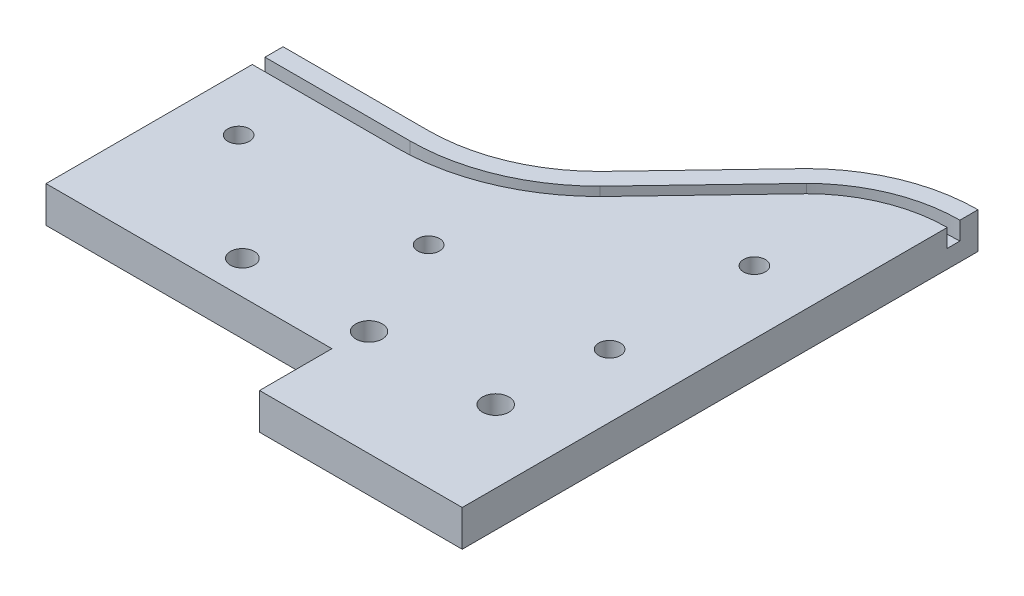
from build123d import *

# Parameters (mm, degrees)
EXTRUDE_1_DEPTH      = 20
CUT_EXTRUDE_1_DEPTH  = 10
SKETCH_4_W           = 45
SKETCH_4_H           = 90
CUT_EXTRUDE_2_DEPTH  = 5
SKETCH_5_W           = 112
SKETCH_5_H           = 20
EXTRUDE_2_DEPTH      = 40
CUT_EXTRUDE_3_REACH  = 1227.871
SKETCH_6_R           = 6
SKETCH_6_R_2         = 5
CUT_EXTRUDE_4_REACH  = 1228.116
SKETCH_7_R           = 7.332886018
SKETCH_7_R_2         = 7.301331484
SKETCH_7_R_3         = 6.603217824
SKETCH_24_R          = 6
CUT_EXTRUDE_21_DEPTH = 25


with BuildPart() as part:
    # 草图1 → 凸台-拉伸1 (new body)
    with BuildSketch(Plane(origin=(0, 0, 0), x_dir=(1, 0, 0), z_dir=(0, 1, 0))):
        with BuildLine():
            Line((-190, -173.659488393), (0, -173.659488393))
            Line((0, -173.659488393), (0, 71.340511607))
            ThreePointArc((0, 71.340511607), (-36.354926075, 64.109067196), (-67.175144213, 43.51565582))
            add(Edge.make_bspline(
                [(-122.824855787, -14.834632605), (-95, 14.340511607), (-67.175144213, 43.51565582)],
                knots=[0, 0, 0, 1, 1, 1], degree=2))
            ThreePointArc((-122.824855787, -14.834632605), (-153.645073925, -35.428043981), (-190, -42.659488393))
            Line((-190, -42.659488393), (-270, -42.659488393))
            Line((-270, -42.659488393), (-270, -173.659488393))
            Line((-270, -173.659488393), (-190, -173.659488393))
        make_face()
    extrude(amount=EXTRUDE_1_DEPTH)

    # 草图2 → 切除-拉伸1 (cut)
    with BuildSketch(Plane(origin=(0, 20, 0), x_dir=(1, 0, 0), z_dir=(0, 1, 0))):
        with BuildLine():
            Line((-270, -52.659488393), (-190, -52.659488393))
            ThreePointArc((-190, -52.659488393), (-149.762170559, -44.64359576), (-115.668000558, -21.819813762))
            Line((-115.668000558, -21.819813762), (-60.022606457, 36.52594767))
            ThreePointArc((-60.022606457, 36.52594767), (-32.474897495, 54.892284551), (0, 61.340511607))
            Line((0, 61.340511607), (0, 54.340511607))
            ThreePointArc((0, 54.340511607), (-29.760862596, 48.439686759), (-55.01881141, 31.630025903))
            Line((-55.01881141, 31.630025903), (-110.655962205, -26.707092192))
            ThreePointArc((-110.655962205, -26.707092192), (-147.042646878, -51.093843482), (-190, -59.659488393))
            Line((-190, -59.659488393), (-270, -59.659488393))
            Line((-270, -59.659488393), (-270, -52.659488393))
        make_face()
    extrude(amount=-CUT_EXTRUDE_1_DEPTH, mode=Mode.SUBTRACT)

    # 草图4 → 切除-拉伸2 (cut)
    with BuildSketch(Plane.XZ):
        with Locations((-247.5, 99.659488393)):
            Rectangle(SKETCH_4_W, SKETCH_4_H)
    extrude(amount=-CUT_EXTRUDE_2_DEPTH, mode=Mode.SUBTRACT)

    # 草图5 → 凸台-拉伸2 (add)
    with BuildSketch(Plane.XY.offset(173.659488393)):
        with Locations((-56, 10)):
            Rectangle(SKETCH_5_W, SKETCH_5_H)
    extrude(amount=EXTRUDE_2_DEPTH)

    # 切除-拉伸3: up to this face of the body (flat: up to its plane)
    cut_extrude_3_end = Plane(part.part.faces().sort_by_distance((-99.039367246, 0, 91.650022184))[0])
    # 草图6 → 切除-拉伸3 (cut, up to the picked face)
    with BuildSketch(Plane(origin=(600.126281628, 25, -649.482989384), x_dir=(0, 0, -1), z_dir=(0, 1, 0)), mode=Mode.PRIVATE) as cut_extrude_3_sk1:
        with Locations(Location((-666.704267343, 635.126281628, 0), (0, 0, 180))):
            Circle(SKETCH_6_R)
    cut_extrude_3_tool1 = split(extrude(cut_extrude_3_sk1.sketch, amount=-CUT_EXTRUDE_3_REACH, mode=Mode.PRIVATE), bisect_by=cut_extrude_3_end, keep=Keep.BOTH, mode=Mode.PRIVATE)
    # 草图6 → 切除-拉伸3 (cut, up to the picked face)
    with BuildSketch(Plane(origin=(600.126281628, 25, -649.482989384), x_dir=(0, 0, -1), z_dir=(0, 1, 0)), mode=Mode.PRIVATE) as cut_extrude_3_sk2:
        with Locations(Location((-746.704267343, 635.126281628, 0), (0, 0, 180))):
            Circle(SKETCH_6_R_2)
    cut_extrude_3_tool2 = split(extrude(cut_extrude_3_sk2.sketch, amount=-CUT_EXTRUDE_3_REACH, mode=Mode.PRIVATE), bisect_by=cut_extrude_3_end, keep=Keep.BOTH, mode=Mode.PRIVATE)
    # 草图6 → 切除-拉伸3 (cut, up to the picked face)
    with BuildSketch(Plane(origin=(600.126281628, 25, -649.482989384), x_dir=(0, 0, -1), z_dir=(0, 1, 0)), mode=Mode.PRIVATE) as cut_extrude_3_sk3:
        with Locations(Location((-746.704267343, 840.126281628, 0), (0, 0, 180))):
            Circle(SKETCH_6_R)
    cut_extrude_3_tool3 = split(extrude(cut_extrude_3_sk3.sketch, amount=-CUT_EXTRUDE_3_REACH, mode=Mode.PRIVATE), bisect_by=cut_extrude_3_end, keep=Keep.BOTH, mode=Mode.PRIVATE)
    # 草图6 → 切除-拉伸3 (cut, up to the picked face)
    with BuildSketch(Plane(origin=(600.126281628, 25, -649.482989384), x_dir=(0, 0, -1), z_dir=(0, 1, 0)), mode=Mode.PRIVATE) as cut_extrude_3_sk4:
        with Locations(Location((-746.704267343, 735.126281628, 0), (0, 0, 180))):
            Circle(SKETCH_6_R)
    cut_extrude_3_tool4 = split(extrude(cut_extrude_3_sk4.sketch, amount=-CUT_EXTRUDE_3_REACH, mode=Mode.PRIVATE), bisect_by=cut_extrude_3_end, keep=Keep.BOTH, mode=Mode.PRIVATE)
    add(cut_extrude_3_tool1.solids().sort_by(Axis((-35, 25, 17.221278), (0, -1, 0)))[0], mode=Mode.SUBTRACT)
    add(cut_extrude_3_tool2.solids().sort_by(Axis((-35, 25, 97.221278), (0, -1, 0)))[0], mode=Mode.SUBTRACT)
    add(cut_extrude_3_tool3.solids().sort_by(Axis((-240, 25, 97.221278), (0, -1, 0)))[0], mode=Mode.SUBTRACT)
    add(cut_extrude_3_tool4.solids().sort_by(Axis((-135, 25, 97.221278), (0, -1, 0)))[0], mode=Mode.SUBTRACT)

    # 草图7 → 切除-拉伸4 (cut, up to next)
    with BuildSketch(Plane(origin=(600.126281628, 35, -649.482989384), x_dir=(0, 0, -1), z_dir=(0, 1, 0)), mode=Mode.PRIVATE) as cut_extrude_4_sk1:
        with Locations(Location((-804.642477777, 640.126281628, 0), (0, 0, 180))):
            Circle(SKETCH_7_R)
    cut_extrude_4_tool1 = extrude(cut_extrude_4_sk1.sketch, amount=-CUT_EXTRUDE_4_REACH, mode=Mode.PRIVATE) & part.part
    # 草图7 → 切除-拉伸4 (cut, up to next)
    with BuildSketch(Plane(origin=(600.126281628, 35, -649.482989384), x_dir=(0, 0, -1), z_dir=(0, 1, 0)), mode=Mode.PRIVATE) as cut_extrude_4_sk2:
        with Locations(Location((-804.642477777, 710.126281628, 0), (0, 0, 180))):
            Circle(SKETCH_7_R_2)
    cut_extrude_4_tool2 = extrude(cut_extrude_4_sk2.sketch, amount=-CUT_EXTRUDE_4_REACH, mode=Mode.PRIVATE) & part.part
    # 草图7 → 切除-拉伸4 (cut, up to next)
    with BuildSketch(Plane(origin=(600.126281628, 35, -649.482989384), x_dir=(0, 0, -1), z_dir=(0, 1, 0)), mode=Mode.PRIVATE) as cut_extrude_4_sk3:
        with Locations(Location((-804.642477777, 780.126281628, 0), (0, 0, 180))):
            Circle(SKETCH_7_R_3)
    cut_extrude_4_tool3 = extrude(cut_extrude_4_sk3.sketch, amount=-CUT_EXTRUDE_4_REACH, mode=Mode.PRIVATE) & part.part
    add(cut_extrude_4_tool1.solids().sort_by_distance((-40, 35, 155.159488))[0], mode=Mode.SUBTRACT)
    add(cut_extrude_4_tool2.solids().sort_by_distance((-110, 35, 155.159488))[0], mode=Mode.SUBTRACT)
    add(cut_extrude_4_tool3.solids().sort_by_distance((-180, 35, 155.159488))[0], mode=Mode.SUBTRACT)

    # 草图24 → 切除-拉伸21 (cut)
    with BuildSketch(Plane(origin=(600.126281628, 25, -649.482989384), x_dir=(0, 0, -1), z_dir=(0, 1, 0))):
        with Locations(Location((-666.704267343, 635.126281628, 0), (0, 0, 180))):
            Circle(SKETCH_24_R)
        with Locations(Location((-746.704267343, 635.126281628, 0), (0, 0, 180))):
            Circle(SKETCH_24_R)
        with Locations(Location((-746.704267343, 840.126281628, 0), (0, 0, 180))):
            Circle(SKETCH_24_R)
        with Locations(Location((-746.704267343, 735.126281628, 0), (0, 0, 180))):
            Circle(SKETCH_24_R)
    extrude(amount=-CUT_EXTRUDE_21_DEPTH, mode=Mode.SUBTRACT)


solid = part.part
